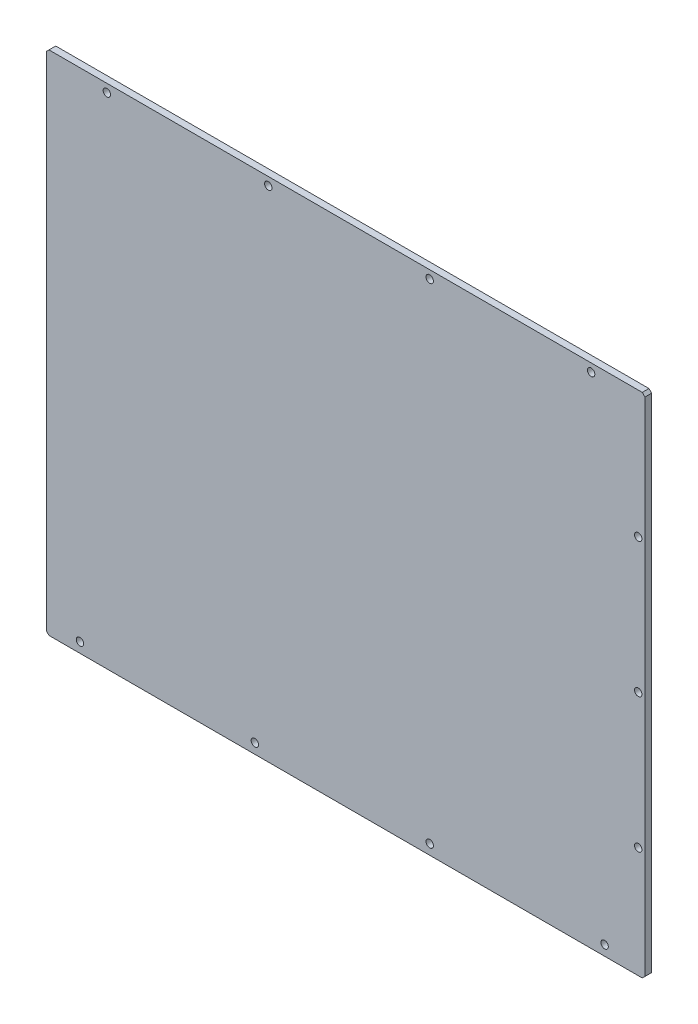
from build123d import *

# Parameters (mm, degrees)
SKETCH1_W            = 445
SKETCH1_H            = 377
BOSS_EXTRUDE1_DEPTH  = 5
M5_CLEARANCE_HOLE1_D = 5.5
FILLET1_SIZE         = 2


with BuildPart() as part:
    # Sketch1 → Boss-Extrude1 (new body)
    with BuildSketch(Plane.XY):
        Rectangle(SKETCH1_W, SKETCH1_H)
    extrude(amount=BOSS_EXTRUDE1_DEPTH)

    # M5 Clearance Hole1 (through all)
    with Locations(Plane.XY.offset(5)):
        with Locations((-177.5, 182.5), (-57.5, 182.5), (62.5, 182.5), (182.5, 182.5), (-197.5, -181), (-67.5, -181), (62.5, -181), (192.5, -181), (217.5, -106), (217.5, -6), (217.5, 94)):
            Hole(M5_CLEARANCE_HOLE1_D / 2)

    # Fillet1
    fillet1_edges = [part.edges().sort_by_distance(p)[0] for p in [
        (222.5, -188.5, 2.5),
        (-222.5, -188.5, 2.5),
        (-222.5, 188.5, 2.5),
        (222.5, 188.5, 2.5),
    ]]
    chamfer(fillet1_edges, length=FILLET1_SIZE)


solid = part.part
